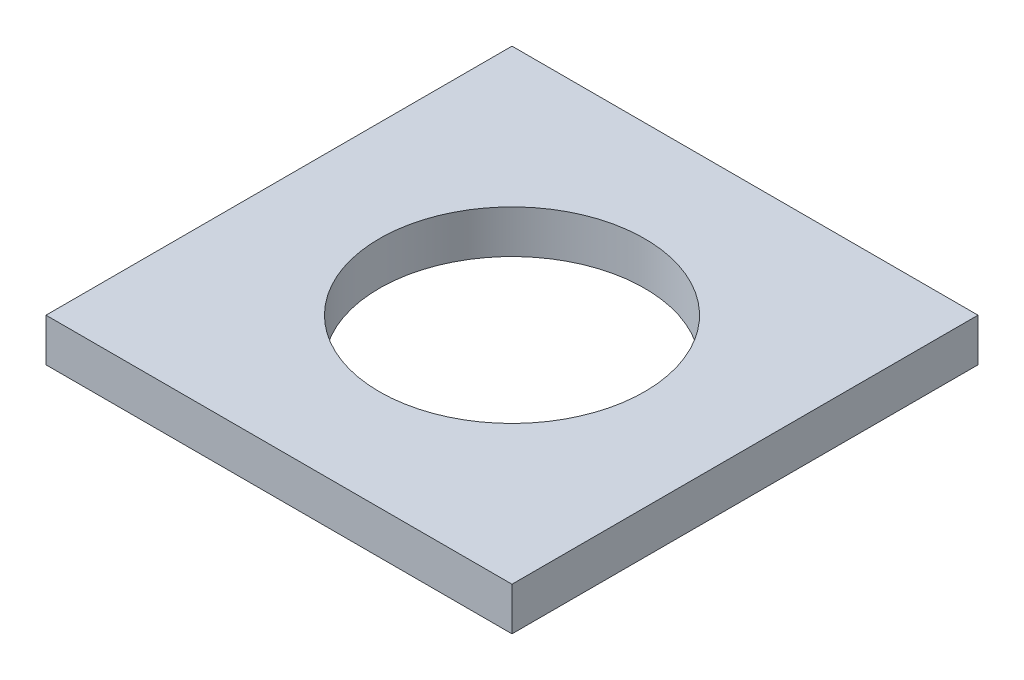
SolidWorks part; units mm, degrees
material "Q235A "
ref_plane "Front Plane" through (0, 0, 0) normal (0, 0, 1) x (1, 0, 0)
ref_plane "Top Plane" through (0, 0, 0) normal (0, 1, 0) x (1, 0, 0)
ref_plane "Right Plane" through (0, 0, 0) normal (1, 0, 0) x (0, 0, -1)
sketch "Sketch2" plane through (0, 0, 0) normal (0, 1, 0) x (1, 0, 0)
  line L1 (-32.5, 32.5) -> (32.5, 32.5)
  line L2 (-32.5, 32.5) -> (-32.5, -32.5)
  line L3 (-32.5, -32.5) -> (32.5, -32.5)
  line L4 (32.5, 32.5) -> (32.5, -32.5)
  circle A0 centre (0, 0) radius 18.5
  dimension "D5" = 37
  dimension "D1" = 65
  dimension "D2" = 65
  dimension "D3" = 32.5
  dimension "D4" = 32.5
extrude "Boss-Extrude1" add sketch "Sketch2" along normal mid plane 6
